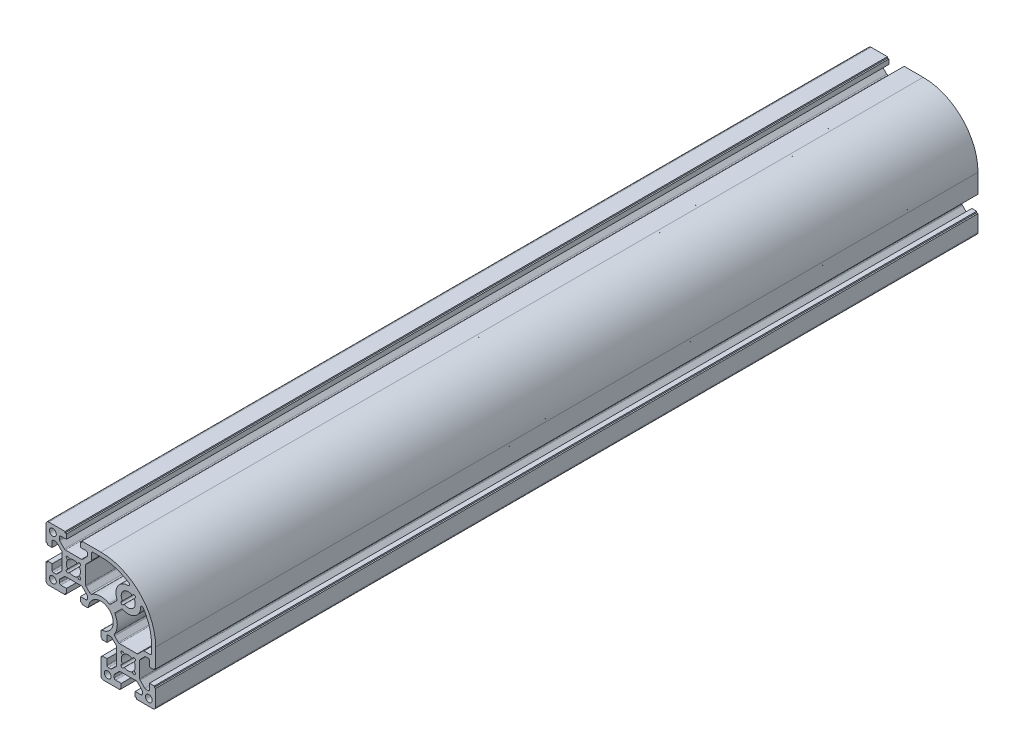
from build123d import *

# Parameters (mm, degrees)
SKETCH1_R           = 2.5
BOSS_EXTRUDE1_DEPTH = 300


with BuildPart() as part:
    # Sketch1 → Boss-Extrude1 (new, symmetric)
    with BuildSketch(Plane.XY):
        with BuildLine():
            Line((-25.101664165, 35.499999963), (-25.101664165, 38.999999963))
            Line((-25.101664165, 38.999999963), (-26.101664165, 38.999999963))
            Line((-26.101664165, 38.999999963), (-26.101664165, 39.999999963))
            Line((-26.101664165, 39.999999963), (-38.001664165, 39.999999963))
            ThreePointArc((-38.001664165, 39.999999963), (-39.415877728, 39.414213525), (-40.001664165, 37.999999963))
            Line((-40.001664165, 37.999999963), (-40.001664165, 26.099999963))
            Line((-40.001664165, 26.099999963), (-39.001664165, 26.099999963))
            Line((-39.001664165, 26.099999963), (-39.001664165, 25.099999963))
            Line((-39.001664165, 25.099999963), (-35.501664165, 25.099999963))
            Line((-35.501664165, 25.099999963), (-35.501664165, 29.249999963))
            ThreePointArc((-35.501664165, 29.249999963), (-35.208770946, 29.957106744), (-34.501664165, 30.249999963))
            Line((-34.501664165, 30.249999963), (-32.786877728, 30.249999963))
            ThreePointArc((-32.786877728, 30.249999963), (-32.4041943, 30.173879497), (-32.079770954, 29.957106751))
            Line((-32.079770954, 29.957106751), (-28.694557384, 26.571893181))
            ThreePointArc((-28.694557384, 26.571893181), (-28.477784633, 26.247469833), (-28.401664165, 25.8647864))
            Line((-28.401664165, 25.8647864), (-28.401664165, 14.136213572))
            ThreePointArc((-28.401664165, 14.136213572), (-28.477756377, 13.753598361), (-28.694452964, 13.429211226))
            Line((-28.694452964, 13.429211226), (-32.079666506, 10.042997621))
            ThreePointArc((-32.079666506, 10.042997621), (-32.404126062, 9.826148689), (-32.786877723, 9.749999963))
            Line((-32.786877723, 9.749999963), (-34.501664165, 9.749999963))
            ThreePointArc((-34.501664165, 9.749999963), (-35.208770946, 10.042893181), (-35.501664165, 10.749999963))
            Line((-35.501664165, 10.749999963), (-35.501664165, 14.899999963))
            Line((-35.501664165, 14.899999963), (-39.001664165, 14.899999963))
            Line((-39.001664165, 14.899999963), (-39.001664165, 13.899999963))
            Line((-39.001664165, 13.899999963), (-40.001664165, 13.899999963))
            Line((-40.001664165, 13.899999963), (-40.001664165, 1.999999963))
            ThreePointArc((-40.001664165, 1.999999963), (-39.415877728, 0.5857864), (-38.001664165, -3.7e-08))
            Line((-38.001664165, -3.7e-08), (-26.101664165, -3.7e-08))
            Line((-26.101664165, -3.7e-08), (-26.101664165, 0.999999963))
            Line((-26.101664165, 0.999999963), (-25.101664165, 0.999999963))
            Line((-25.101664165, 0.999999963), (-25.101664165, 4.499999963))
            Line((-25.101664165, 4.499999963), (-29.251664165, 4.499999963))
            ThreePointArc((-29.251664165, 4.499999963), (-29.958770946, 4.792893181), (-30.251664165, 5.499999963))
            Line((-30.251664165, 5.499999963), (-30.251664165, 7.214786416))
            ThreePointArc((-30.251664165, 7.214786416), (-30.175515439, 7.597538063), (-29.958666518, 7.92199761))
            Line((-29.958666518, 7.92199761), (-26.572452898, 11.307211168))
            ThreePointArc((-26.572452898, 11.307211168), (-26.248065773, 11.523907748), (-25.865450576, 11.599999963))
            Line((-25.865450576, 11.599999963), (-14.136877728, 11.599999963))
            ThreePointArc((-14.136877728, 11.599999963), (-13.7541943, 11.523879497), (-13.429770954, 11.307106751))
            Line((-13.429770954, 11.307106751), (-10.044557384, 7.921893181))
            ThreePointArc((-10.044557384, 7.921893181), (-9.827784633, 7.597469833), (-9.751664165, 7.2147864))
            Line((-9.751664165, 7.2147864), (-9.751664165, 5.499999963))
            ThreePointArc((-9.751664165, 5.499999963), (-10.044557384, 4.792893181), (-10.751664165, 4.499999963))
            Line((-10.751664165, 4.499999963), (-14.901664165, 4.499999963))
            Line((-14.901664165, 4.499999963), (-14.901664165, 0.999999963))
            Line((-14.901664165, 0.999999963), (-13.901664165, 0.999999963))
            Line((-13.901664165, 0.999999963), (-13.901664165, -3.7e-08))
            Line((-13.901664165, -3.7e-08), (-9.951651602, -3.7e-08))
            ThreePointArc((-9.951651602, -3.7e-08), (-9.280830978, 0.258380323), (-8.956664103, 0.900000582))
            ThreePointArc((-8.956664103, 0.900000582), (6.362171395, 6.363835063), (0.898335806, -8.95500004))
            ThreePointArc((0.898335806, -8.95500004), (0.256715976, -9.279167092), (-0.001664165, -9.949987475))
            Line((-0.001664165, -9.949987475), (-0.001664165, -13.900000037))
            Line((-0.001664165, -13.900000037), (0.998335835, -13.900000037))
            Line((0.998335835, -13.900000037), (0.998335835, -14.900000037))
            Line((0.998335835, -14.900000037), (4.498335835, -14.900000037))
            Line((4.498335835, -14.900000037), (4.498335835, -10.750000037))
            ThreePointArc((4.498335835, -10.750000037), (4.791229054, -10.042893256), (5.498335835, -9.750000037))
            Line((5.498335835, -9.750000037), (7.213122272, -9.750000037))
            ThreePointArc((7.213122272, -9.750000037), (7.5958057, -9.826120503), (7.920229046, -10.042893249))
            Line((7.920229046, -10.042893249), (11.305442616, -13.428106819))
            ThreePointArc((11.305442616, -13.428106819), (11.522215367, -13.752530167), (11.598335835, -14.1352136))
            Line((11.598335835, -14.1352136), (11.598335835, -25.863786428))
            ThreePointArc((11.598335835, -25.863786428), (11.522243623, -26.246401639), (11.305547036, -26.570788774))
            Line((11.305547036, -26.570788774), (7.920333494, -29.957002379))
            ThreePointArc((7.920333494, -29.957002379), (7.595873938, -30.173851311), (7.213122277, -30.250000037))
            Line((7.213122277, -30.250000037), (5.498335835, -30.250000037))
            ThreePointArc((5.498335835, -30.250000037), (4.791229054, -29.957106819), (4.498335835, -29.250000037))
            Line((4.498335835, -29.250000037), (4.498335835, -25.100000037))
            Line((4.498335835, -25.100000037), (0.998335835, -25.100000037))
            Line((0.998335835, -25.100000037), (0.998335835, -26.100000037))
            Line((0.998335835, -26.100000037), (-0.001664165, -26.100000037))
            Line((-0.001664165, -26.100000037), (-0.001664165, -38.000000037))
            ThreePointArc((-0.001664165, -38.000000037), (0.584122272, -39.4142136), (1.998335835, -40.000000037))
            Line((1.998335835, -40.000000037), (13.898335835, -40.000000037))
            Line((13.898335835, -40.000000037), (13.898335835, -39.000000037))
            Line((13.898335835, -39.000000037), (14.898335835, -39.000000037))
            Line((14.898335835, -39.000000037), (14.898335835, -35.500000037))
            Line((14.898335835, -35.500000037), (10.748335835, -35.500000037))
            ThreePointArc((10.748335835, -35.500000037), (10.041229054, -35.207106819), (9.748335835, -34.500000037))
            Line((9.748335835, -34.500000037), (9.748335835, -32.785213584))
            ThreePointArc((9.748335835, -32.785213584), (9.824484561, -32.402461937), (10.041333482, -32.07800239))
            Line((10.041333482, -32.07800239), (13.427547102, -28.692788832))
            ThreePointArc((13.427547102, -28.692788832), (13.751934227, -28.476092252), (14.134549424, -28.400000037))
            Line((14.134549424, -28.400000037), (25.863122272, -28.400000037))
            ThreePointArc((25.863122272, -28.400000037), (26.2458057, -28.476120503), (26.570229046, -28.692893249))
            Line((26.570229046, -28.692893249), (29.955442616, -32.078106819))
            ThreePointArc((29.955442616, -32.078106819), (30.172215367, -32.402530167), (30.248335835, -32.7852136))
            Line((30.248335835, -32.7852136), (30.248335835, -34.500000037))
            ThreePointArc((30.248335835, -34.500000037), (29.955442616, -35.207106819), (29.248335835, -35.500000037))
            Line((29.248335835, -35.500000037), (25.098335835, -35.500000037))
            Line((25.098335835, -35.500000037), (25.098335835, -39.000000037))
            Line((25.098335835, -39.000000037), (26.098335835, -39.000000037))
            Line((26.098335835, -39.000000037), (26.098335835, -40.000000037))
            Line((26.098335835, -40.000000037), (37.998335835, -40.000000037))
            ThreePointArc((37.998335835, -40.000000037), (39.412549397, -39.4142136), (39.998335835, -38.000000037))
            Line((39.998335835, -38.000000037), (39.998335835, -26.100000037))
            Line((39.998335835, -26.100000037), (38.998335835, -26.100000037))
            Line((38.998335835, -26.100000037), (38.998335835, -25.100000037))
            Line((38.998335835, -25.100000037), (35.498335835, -25.100000037))
            Line((35.498335835, -25.100000037), (35.498335835, -29.250000037))
            ThreePointArc((35.498335835, -29.250000037), (35.205442616, -29.957106819), (34.498335835, -30.250000037))
            Line((34.498335835, -30.250000037), (32.784549397, -30.250000037))
            ThreePointArc((32.784549397, -30.250000037), (32.40186597, -30.173879572), (32.077442623, -29.957106826))
            Line((32.077442623, -29.957106826), (28.691229054, -26.570893256))
            ThreePointArc((28.691229054, -26.570893256), (28.474456302, -26.246469907), (28.398335835, -25.863786475))
            Line((28.398335835, -25.863786475), (28.398335835, -14.135213584))
            ThreePointArc((28.398335835, -14.135213584), (28.474484561, -13.752461937), (28.691333482, -13.42800239))
            Line((28.691333482, -13.42800239), (32.077547102, -10.042788832))
            ThreePointArc((32.077547102, -10.042788832), (32.401934227, -9.826092252), (32.784549424, -9.750000037))
            Line((32.784549424, -9.750000037), (34.498335835, -9.750000037))
            ThreePointArc((34.498335835, -9.750000037), (35.205442616, -10.042893256), (35.498335835, -10.750000037))
            Line((35.498335835, -10.750000037), (35.498335835, -14.900000037))
            Line((35.498335835, -14.900000037), (38.998335835, -14.900000037))
            Line((38.998335835, -14.900000037), (38.998335835, -13.900000037))
            Line((38.998335835, -13.900000037), (39.998335835, -13.900000037))
            Line((39.998335835, -13.900000037), (39.998335835, -3.7e-08))
            ThreePointArc((39.998335835, -3.7e-08), (28.282607082, 28.28427121), (-0.001664165, 39.999999963))
            Line((-0.001664165, 39.999999963), (-13.901664165, 39.999999963))
            Line((-13.901664165, 39.999999963), (-13.901664165, 38.999999963))
            Line((-13.901664165, 38.999999963), (-14.901664165, 38.999999963))
            Line((-14.901664165, 38.999999963), (-14.901664165, 35.499999963))
            Line((-14.901664165, 35.499999963), (-10.751664165, 35.499999963))
            ThreePointArc((-10.751664165, 35.499999963), (-10.044557384, 35.207106744), (-9.751664165, 34.499999963))
            Line((-9.751664165, 34.499999963), (-9.751664165, 32.786213572))
            ThreePointArc((-9.751664165, 32.786213572), (-9.827756377, 32.403598361), (-10.044452964, 32.079211226))
            Line((-10.044452964, 32.079211226), (-13.429666506, 28.692997621))
            ThreePointArc((-13.429666506, 28.692997621), (-13.754126062, 28.476148689), (-14.136877723, 28.399999963))
            Line((-14.136877723, 28.399999963), (-25.865450603, 28.399999963))
            ThreePointArc((-25.865450603, 28.399999963), (-26.24813403, 28.476120428), (-26.572557377, 28.692893174))
            Line((-26.572557377, 28.692893174), (-29.958770946, 32.079106744))
            ThreePointArc((-29.958770946, 32.079106744), (-30.175543698, 32.403530093), (-30.251664165, 32.786213525))
            Line((-30.251664165, 32.786213525), (-30.251664165, 34.499999963))
            ThreePointArc((-30.251664165, 34.499999963), (-29.958770946, 35.207106744), (-29.251664165, 35.499999963))
            Line((-29.251664165, 35.499999963), (-25.101664165, 35.499999963))
        make_face()
        with Locations((-35.001664165, 34.999999963)):
            Circle(SKETCH1_R, mode=Mode.SUBTRACT)
        with Locations((4.998335835, -35.000000037)):
            Circle(SKETCH1_R, mode=Mode.SUBTRACT)
        with Locations((34.998335835, -35.000000037)):
            Circle(SKETCH1_R, mode=Mode.SUBTRACT)
        with Locations((-35.001664165, 4.999999963)):
            Circle(SKETCH1_R, mode=Mode.SUBTRACT)
        with BuildLine():
            Line((-23.608664165, 14.978999963), (-22.830664165, 15.756999963))
            ThreePointArc((-22.830664165, 15.756999963), (-20.001664165, 14.900437131), (-17.172664165, 15.756999963))
            Line((-17.172664165, 15.756999963), (-16.394414165, 14.978749963))
            ThreePointArc((-16.394414165, 14.978749963), (-14.979914165, 14.978749963), (-14.979914165, 16.393249963))
            Line((-14.979914165, 16.393249963), (-15.757664165, 17.170999963))
            ThreePointArc((-15.757664165, 17.170999963), (-14.901101333, 19.999999963), (-15.757664165, 22.828999963))
            Line((-15.757664165, 22.828999963), (-14.979914165, 23.606749963))
            ThreePointArc((-14.979914165, 23.606749963), (-14.980209003, 25.020848355), (-16.394307335, 25.021356334))
            Line((-16.394307335, 25.021356334), (-17.172664165, 24.243999963))
            ThreePointArc((-17.172664165, 24.243999963), (-20.001664165, 25.100562794), (-22.830664165, 24.243999963))
            Line((-22.830664165, 24.243999963), (-23.608664165, 25.020999963))
            ThreePointArc((-23.608664165, 25.020999963), (-25.010482741, 25.008818538), (-25.022664165, 23.606999963))
            Line((-25.022664165, 23.606999963), (-24.244664165, 22.828999963))
            ThreePointArc((-24.244664165, 22.828999963), (-25.101226997, 19.999999963), (-24.244664165, 17.170999963))
            Line((-24.244664165, 17.170999963), (-25.022664165, 16.392999963))
            ThreePointArc((-25.022664165, 16.392999963), (-25.010482741, 14.991181387), (-23.608664165, 14.978999963))
        make_face(mode=Mode.SUBTRACT)
        with BuildLine():
            Line((27.170229054, -10.707106819), (30.834442623, -7.042893249))
            ThreePointArc((30.834442623, -7.042893249), (31.15886597, -6.826120503), (31.541549397, -6.750000037))
            Line((31.541549397, -6.750000037), (35.998335835, -6.750000037))
            ThreePointArc((35.998335835, -6.750000037), (36.705442616, -6.457106819), (36.998335835, -5.750000037))
            Line((36.998335835, -5.750000037), (36.998335835, 0.000697362))
            ThreePointArc((36.998335835, 0.000697362), (35.445239791, 10.60810044), (30.916335835, 20.324999962))
            ThreePointArc((30.916335835, 20.324999962), (29.799075151, 20.736004824), (29.080335835, 19.786999962))
            ThreePointArc((29.080335835, 19.786999962), (24.850415615, 12.255980052), (16.227335835, 11.754999963))
            ThreePointArc((16.227335835, 11.754999963), (15.6287507, 11.836373329), (15.092524179, 11.558188307))
            Line((15.092524179, 11.558188307), (10.619768343, 7.08543247))
            ThreePointArc((10.619768343, 7.08543247), (10.336172335, 6.514369859), (10.455335841, 5.887999952))
            ThreePointArc((10.455335841, 5.887999952), (11.989509024, -0.474073057), (9.957335837, -6.695000034))
            ThreePointArc((9.957335837, -6.695000034), (9.792012525, -7.349472347), (10.080219791, -7.959883993))
            Line((10.080219791, -7.959883993), (12.827442623, -10.707106826))
            ThreePointArc((12.827442623, -10.707106826), (13.15186597, -10.923879572), (13.534549397, -11.000000037))
            Line((13.534549397, -11.000000037), (26.463122269, -11.000000037))
            ThreePointArc((26.463122269, -11.000000037), (26.845805703, -10.923879571), (27.170229054, -10.707106819))
        make_face(mode=Mode.SUBTRACT)
        with BuildLine():
            Line((7.084408086, 10.621072214), (11.560007531, 15.096671659))
            ThreePointArc((11.560007531, 15.096671659), (11.836402753, 15.622881137), (11.765335835, 16.212999962))
            ThreePointArc((11.765335835, 16.212999962), (12.450348188, 24.815561391), (20.059335835, 28.886999963))
            ThreePointArc((20.059335835, 28.886999963), (21.024529702, 29.591619698), (20.625335826, 30.717999927))
            ThreePointArc((20.625335826, 30.717999927), (10.780398907, 35.394674694), (0, 36.999999963))
            Line((0, 36.999999963), (-5.751664165, 36.999999963))
            ThreePointArc((-5.751664165, 36.999999963), (-6.458770946, 36.707106744), (-6.751664165, 35.999999963))
            Line((-6.751664165, 35.999999963), (-6.751664165, 31.543213528))
            ThreePointArc((-6.751664165, 31.543213528), (-6.827784632, 31.160530094), (-7.044557384, 30.836106744))
            Line((-7.044557384, 30.836106744), (-10.708770954, 27.171893174))
            ThreePointArc((-10.708770954, 27.171893174), (-10.9255437, 26.847469828), (-11.001664165, 26.4647864))
            Line((-11.001664165, 26.4647864), (-11.001664165, 13.536213528))
            ThreePointArc((-11.001664165, 13.536213528), (-10.925543698, 13.153530094), (-10.708770946, 12.829106744))
            Line((-10.708770946, 12.829106744), (-7.961548122, 10.081883919))
            ThreePointArc((-7.961548122, 10.081883919), (-7.351136483, 9.793676654), (-6.696664174, 9.958999957))
            ThreePointArc((-6.696664174, 9.958999957), (-0.475737185, 11.991173152), (5.886335835, 10.456999963))
            ThreePointArc((5.886335835, 10.456999963), (6.512981785, 10.337426348), (7.084408086, 10.621072214))
        make_face(mode=Mode.SUBTRACT)
        with BuildLine():
            Line((23.588335835, 24.908999963), (22.810335835, 24.130999963))
            ThreePointArc((22.810335835, 24.130999963), (16.376401917, 23.49293388), (15.738335835, 17.058999963))
            Line((15.738335835, 17.058999963), (14.960085813, 16.28074994))
            ThreePointArc((14.960085813, 16.28074994), (14.96008578, 14.866249929), (16.374585791, 14.866249918))
            Line((16.374585791, 14.866249918), (17.152335835, 15.643999963))
            ThreePointArc((17.152335835, 15.643999963), (23.587723937, 16.281521784), (24.224335835, 22.716999963))
            Line((24.224335835, 22.716999963), (25.002335835, 23.494999963))
            ThreePointArc((25.002335835, 23.494999963), (24.99015441, 24.896818538), (23.588335835, 24.908999963))
        make_face(mode=Mode.SUBTRACT)
        with BuildLine():
            Line((16.391335835, -25.021000037), (17.169335835, -24.243000037))
            ThreePointArc((17.169335835, -24.243000037), (19.998335835, -25.099562869), (22.827335835, -24.243000037))
            Line((22.827335835, -24.243000037), (23.605585835, -25.021250037))
            ThreePointArc((23.605585835, -25.021250037), (25.020085835, -25.021250037), (25.020085835, -23.606750037))
            Line((25.020085835, -23.606750037), (24.242335835, -22.829000037))
            ThreePointArc((24.242335835, -22.829000037), (25.098898667, -20.000000037), (24.242335835, -17.171000037))
            Line((24.242335835, -17.171000037), (25.020085835, -16.393250037))
            ThreePointArc((25.020085835, -16.393250037), (25.019790997, -14.979151645), (23.605692665, -14.978643666))
            Line((23.605692665, -14.978643666), (22.827335835, -15.756000037))
            ThreePointArc((22.827335835, -15.756000037), (19.998335835, -14.899437206), (17.169335835, -15.756000037))
            Line((17.169335835, -15.756000037), (16.391335835, -14.979000037))
            ThreePointArc((16.391335835, -14.979000037), (14.989517259, -14.991181462), (14.977335835, -16.393000037))
            Line((14.977335835, -16.393000037), (15.755335835, -17.171000037))
            ThreePointArc((15.755335835, -17.171000037), (14.898773003, -20.000000037), (15.755335835, -22.829000037))
            Line((15.755335835, -22.829000037), (14.977335835, -23.607000037))
            ThreePointArc((14.977335835, -23.607000037), (14.989517259, -25.008818613), (16.391335835, -25.021000037))
        make_face(mode=Mode.SUBTRACT)
    extrude(amount=BOSS_EXTRUDE1_DEPTH, both=True)


solid = part.part
